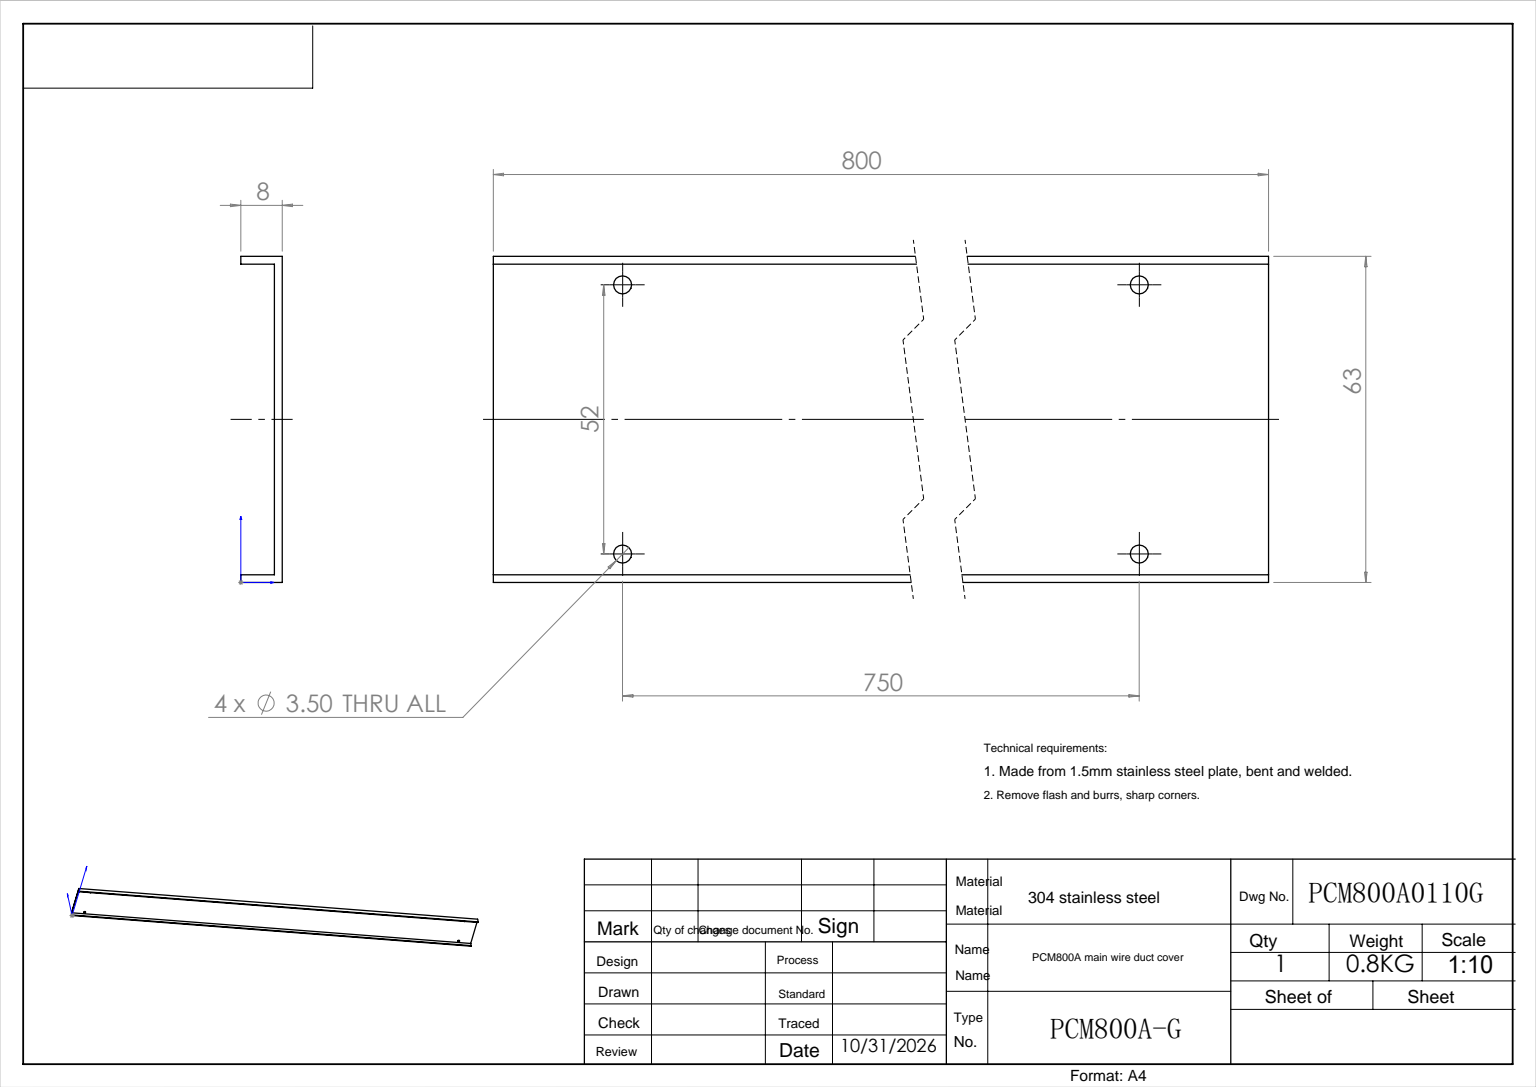
from build123d import *

# Parameters (mm, degrees)
EXTRUDE_1_DEPTH         = 800
HOLE_WIZARD_3_5_3_5_1_D = 3.5


with BuildPart() as part:
    # 草图1 → 拉伸-薄壁1 (new body)
    with BuildSketch(Plane.XY):
        Polygon((0, 0), (8, 0), (8, 63), (0, 63), (0, 61.5), (6.5, 61.5), (6.5, 1.5), (0, 1.5), align=None)
    extrude(amount=EXTRUDE_1_DEPTH)

    # Ø3.5 (3.5) 直径孔1 (through all)
    with Locations(Plane(origin=(8, 0, 0), x_dir=(0, 0, -1), z_dir=(1, 0, 0))):
        with Locations((-775, 57.5), (-25, 57.5)):
            hole_wizard_3_5_3_5_1 = Hole(HOLE_WIZARD_3_5_3_5_1_D / 2)

    # 镜向1: Ø3.5 (3.5) 直径孔1 across plane
    add(hole_wizard_3_5_3_5_1.mirror(Plane(origin=(0, 31.5, 0), x_dir=(0, 0, 1), z_dir=(0, -1, 0))), mode=Mode.SUBTRACT)


solid = part.part
